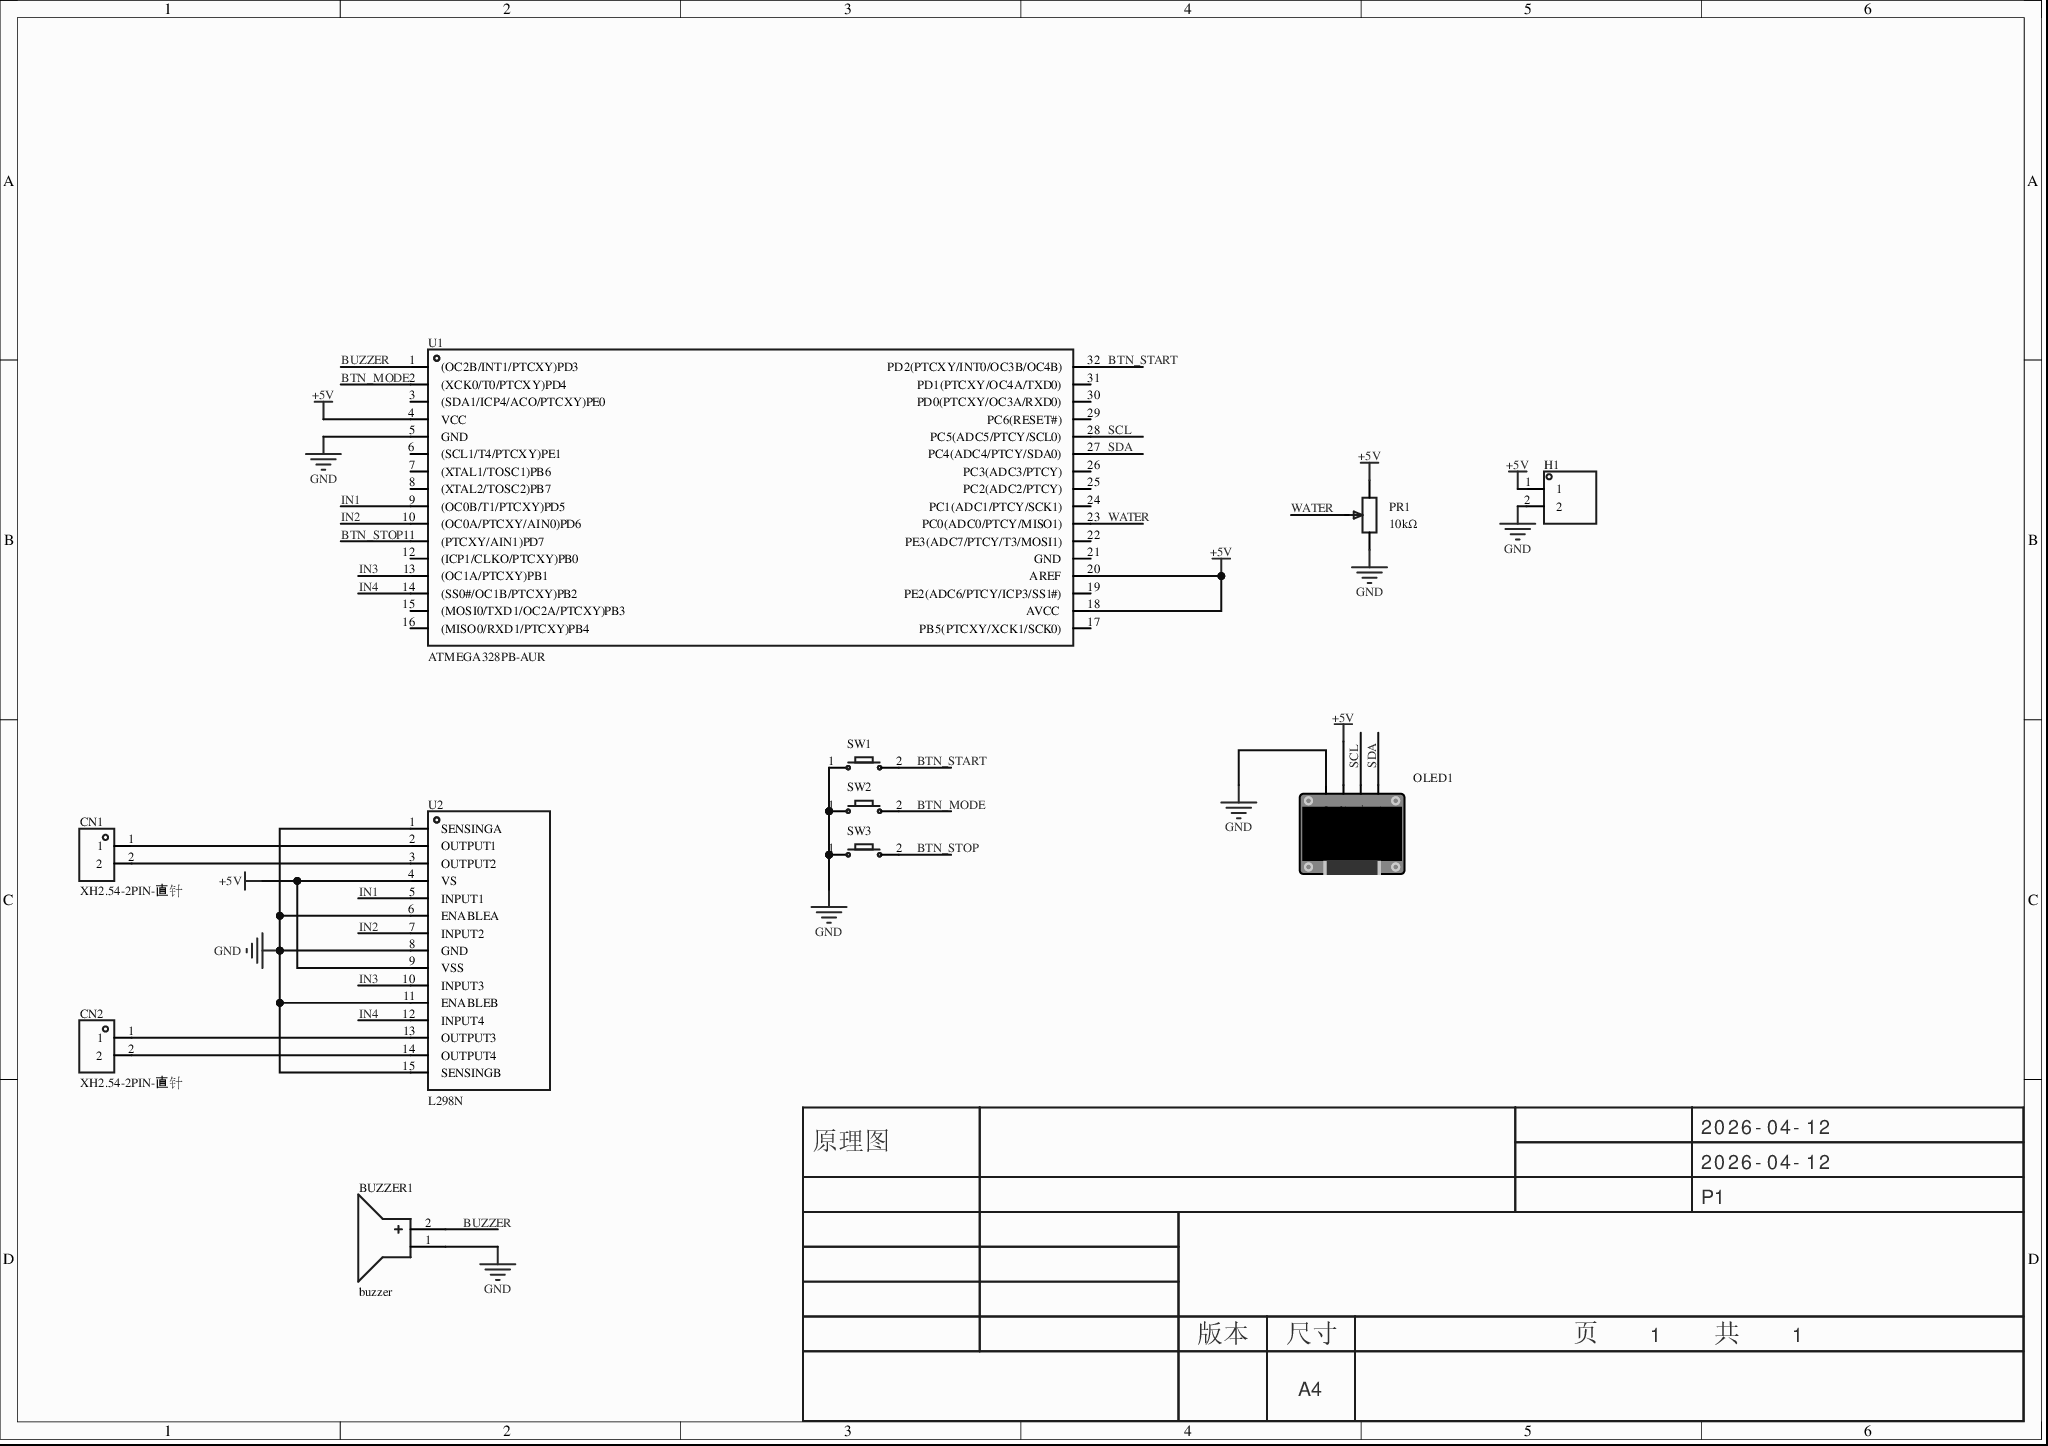
[diagram p0: MISC52152-3.schdoc]
# Altium project MISC52152-2.PrjPcb
1 sheet, 11 parts. Net scope: global (net labels, ports and power ports of the same name join across sheets).
Board file: MISC52152.pcbdoc

## Sheet MISC52152-3.schdoc
size 297 x 209 mm; Version: V1.0; @Project Name: MISC52152; @Update Date: 2026-04-12; @Create Date: 2026-04-12; @Board Name: MISC52152; @Create Time: 20:10:05; @Page Count: 1; @Page No: 1; @Schematic Name: MISC52152; @Update Time: 20:10:05; Size: A4

### Parts
BUZZER1  buzzer  [BUZ-TH_BD12.0-P6.00-D0.9-RD]
CN1  XH2.54-2PIN-直针  [CONN-TH_XH2.54-2P]
CN2  XH2.54-2PIN-直针  [CONN-TH_XH2.54-2P]
H1  (no value)  [HDR-TH_2P-P2.54-V-M-1]
OLED1  (no value)  [0.96OLED_4P]
PR1  10kΩ  [R_3296]
SW1  (no value)  [Key_SMD_3x4x2]
SW2  (no value)  [Key_SMD_3x4x2]
SW3  (no value)  [Key_SMD_3x4x2]
U1  ATMEGA328PB-AUR  [TQFP-32_L7.0-W7.0-P0.80-LS9.0-BL]
U2  L298N  [MULTIWATT-15_L19.6-W5.0-P1.27-L]

### Nets
+5V: H1.1 OLED1.2(VCC) PR1.1 U1.4(VCC) U1.18(AVCC) U1.20(AREF) U2.4(VS) U2.9(VSS)
GND: BUZZER1.1(-) H1.2 OLED1.1(GND) PR1.3 SW1.1 SW2.1 SW3.1 U1.5(GND) U2.1(SENSINGA) U2.6(ENABLEA) U2.8(GND) U2.11(ENABLEB) U2.15(SENSINGB)
BTN_MODE: SW2.2 U1.2((XCK0/T0/PTCXY)PD4)
BTN_START: SW1.2 U1.32(PD2(PTCXY/INT0/OC3B/OC4B))
BTN_STOP: SW3.2 U1.11((PTCXY/AIN1)PD7)
BUZZER: BUZZER1.2(+) U1.1((OC2B/INT1/PTCXY)PD3)
IN1: U1.9((OC0B/T1/PTCXY)PD5) U2.5(INPUT1)
IN2: U1.10((OC0A/PTCXY/AIN0)PD6) U2.7(INPUT2)
IN3: U1.13((OC1A/PTCXY)PB1) U2.10(INPUT3)
IN4: U1.14((SS0#/OC1B/PTCXY)PB2) U2.12(INPUT4)
SCL: OLED1.3(SCL) U1.28(PC5(ADC5/PTCY/SCL0))
SDA: OLED1.4(SDA) U1.27(PC4(ADC4/PTCY/SDA0))
WATER: PR1.2 U1.23(PC0(ADC0/PTCY/MISO1))
NetCN1_1: CN1.1 U2.2(OUTPUT1)
NetCN1_2: CN1.2 U2.3(OUTPUT2)
NetCN2_1: CN2.1 U2.13(OUTPUT3)
NetCN2_2: CN2.2 U2.14(OUTPUT4)

Not connected (* = marked no-connect by the designer): U1 3((SDA1/ICP4/ACO/PTCXY)PE0) 6((SCL1/T4/PTCXY)PE1) 7((XTAL1/TOSC1)PB6) 8((XTAL2/TOSC2)PB7) 12((ICP1/CLKO/PTCXY)PB0) 15((MOSI0/TXD1/OC2A/PTCXY)PB3) 16((MISO0/RXD1/PTCXY)PB4) 17(PB5(PTCXY/XCK1/SCK0)) 19(PE2(ADC6/PTCY/ICP3/SS1#)) 21(GND) 22(PE3(ADC7/PTCY/T3/MOSI1)) 24(PC1(ADC1/PTCY/SCK1)) 25(PC2(ADC2/PTCY)) 26(PC3(ADC3/PTCY)) 29(PC6(RESET#)) 30(PD0(PTCXY/OC3A/RXD0)) 31(PD1(PTCXY/OC4A/TXD0))

### Notes on the sheet
- 2026-04-12
- 原理图
- P1
- 版本
- 尺寸
- A4
- 页    1    共    1

### Library data of the parts
BUZZER1 = buzzer: AddInBom: yes; ModelId: af17e4151ed84fc2a628230bf23763630819f05c4eef4c71ace90d822a990e87; ModelTransform: 472.44,472.176,0,270,0,0,0,0,-196.85; Symbol: BUZZER; Device: buzzer; LCSC Part Name: buzzer; SupplierPart: C9900014030; ManufacturerPart: buzzer; Supplier Footprint: buzzer; JLCPCB Part Class: Extended Part; Supplier: LCSC; ConvertToPcb: yes; FootprintName: BUZ-TH_BD12.0-P6.00-D0.9-RD; ModelName: BUZ-TH_BD12.0-P6.00-D0.9-RD
CN1 CN2 = XH2.54-2PIN-直针: AddInBom: yes; ModelId: c3cc11bd8b8748c1ae6bc231aac3a1ff0819f05c4eef4c71ace90d822a990e87; ModelTransform: 296.889,230.315,0,0,0,0,0,26.653,-137.795; Symbol: XH2.54-2PIN-直针; Device: XH2.54-2PIN-直针; LCSC Part Name: XH2.54-2PIN-直针; SupplierPart: C9900011425; ManufacturerPart: XH2.54-2PIN-直针; Supplier Footprint: XH2.54-2PIN; JLCPCB Part Class: Extended Part; Supplier: LCSC; ConvertToPcb: yes; FootprintName: CONN-TH_XH2.54-2P; ModelName: CONN-TH_XH2.54-2P
H1 = HDR-M_2.54_1x2P: Symbol: 210S-1*2P L=11.6MMGold-plated black; ConvertToPcb: yes; ModelId: 79b2e9f2d70a4d68a1b7098f27c6d4c50819f05c4eef4c71ace90d822a990e87; ModelName: HDR-M-2.54_1x2; ModelTransform: 200,100,0,0,0,0,0,0,-118.11; Device: HDR-M_2.54_1x2P; AddInBom: yes; SupplierPart: C124375; Supplier Footprint: 插件; FootprintName: HDR-TH_2P-P2.54-V-M-1
OLED1 = 0.96OLED模块_4P: ConvertToPcb: yes; ModelId: 79c000fdb68d45a296c2e9bedf4f90550819f05c4eef4c71ace90d822a990e87; ModelTransform: 1393.69792,1318.895,0,0,0,0,0,-560.079,-137.795; Symbol: 0.96OLED模块_4P; Device: 0.96OLED模块_4P; AddInBom: yes; FootprintName: 0.96OLED_4P; Supplier Footprint: 插件; ModelName: 0.96OLED_4P
PR1 = R_3296: ConvertToPcb: yes; ModelId: b182808559bb43bda9e7de64b64134cb0819f05c4eef4c71ace90d822a990e87; ModelName: 3296W; ModelTransform: 373.98,188.96,590.49,180,0,0,0,0,-140; Symbol: R_3296; Device: R_3296; AddInBom: yes; Supplier Footprint: 直插; FootprintName: R_3296; Value: 10kΩ
SW1-SW3 = Key_SMD_3x4x2: Symbol: 轻触按键x2; ConvertToPcb: yes; ModelId: 63599cce708d48afbce1b0db003544770819f05c4eef4c71ace90d822a990e87; ModelName: SW-SMD_L4.0-W2.9-H2-LS5.0; ModelTransform: 196.85,114.17,79.13,0,0,0,0,0,0; Device: Key_SMD_3x4x2; AddInBom: yes; Supplier Footprint: SMD; FootprintName: Key_SMD_3x4x2
U1 = ATMEGA328PB-AUR: CPU内核:AVR;CPU最大主频:20MHz;CPU位数:8 Bit;; Manufacturer: MICROCHIP(美国微芯); AddInBom: yes; ModelId: 2f509107a7a846499a7beaa4f6ecf97b0819f05c4eef4c71ace90d822a990e87; ModelName: TQFP-32_L7.0-W7.0-H1.2-LS9.0-P0.80; ModelTransform: 354.98382,354.98386,0,90,0,0,-0.039,0.079,0; CPU Core: AVR; CPU Maximum Speed: 20MHz; Core Size: 8 Bit; Program Storage Size: 32KB; Program Memory Type: FLASH; RAM Size: 2KB; EEPROM: 1KB; Number of I/O: 27; ADC (Bit): 10bit; Oscillator Type: 内置; Voltage - Supply: 1.8V~5.5V; Symbol: ATMEGA328PB-AUR; Device: ATMEGA328PB-AUR; LCSC Part Name: ATMEGA328PB-AUR; SupplierPart: C461612; ManufacturerPart: ATMEGA328PB-AUR; Supplier Footprint: TQFP-32(7x7); JLCPCB Part Class: Extended Part; Datasheet: https://item.szlcsc.com/datasheet/ATMEGA328PB-AUR/466103.html; Supplier: LCSC; ConvertToPcb: yes; FootprintName: TQFP-32_L7.0-W7.0-P0.80-LS9.0-BL; Operating Temperature: -40℃~+85℃
U2 = L298N_C504386: AddInBom: yes; ModelId: 17dbda3c803a45a0ac2c74e6ab5d57900819f05c4eef4c71ace90d822a990e87; ModelTransform: 795.27392,389.3693,0,0,0,0,0,84.646,-137.795; Symbol: L298N_C504386; Device: L298N_C504386; LCSC Part Name: L298N; SupplierPart: C504386; ManufacturerPart: L298N; Supplier Footprint: Multiwatt-15; JLCPCB Part Class: Extended Part; Datasheet: https://atta.szlcsc.com/upload/public/pdf/source/20200327/C504386_BB56E557909DA61C724DC028E8A3599A.pdf; Supplier: LCSC; ConvertToPcb: yes; FootprintName: MULTIWATT-15_L19.6-W5.0-P1.27-L; ModelName: MULTIWATT-15_L19.6-W5.0-P1.27-L